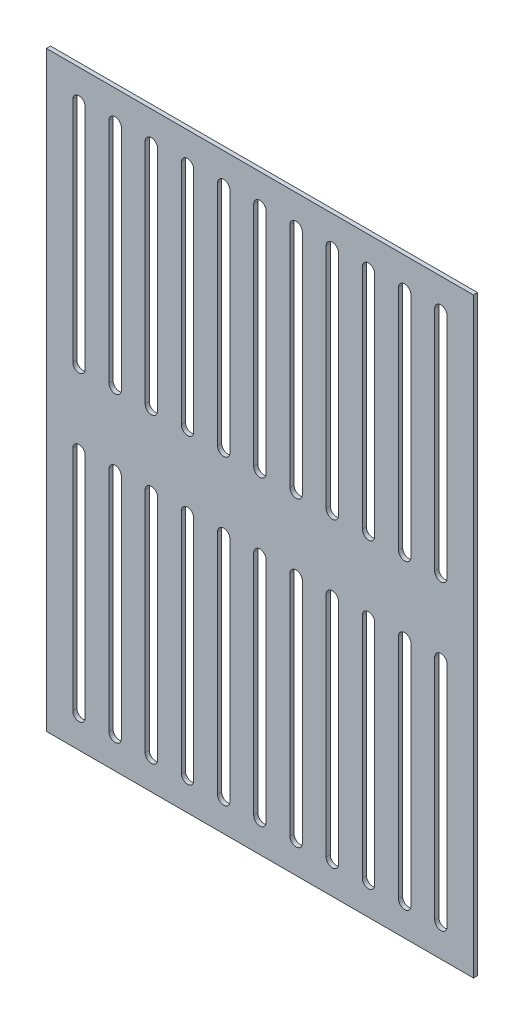
from build123d import *

# Parameters (mm, degrees)
SKETCH1_W           = 413
SKETCH1_H           = 572
BOSS_EXTRUDE1_DEPTH = 4
CUT_EXTRUDE1_DEPTH  = 4


with BuildPart() as part:
    # Sketch1 → Boss-Extrude1 (new body)
    with BuildSketch(Plane.XY):
        Rectangle(SKETCH1_W, SKETCH1_H)
    extrude(amount=BOSS_EXTRUDE1_DEPTH)

    # Sketch2 → Cut-Extrude1 (cut)
    with BuildSketch(Plane.XY.offset(4)):
        with BuildLine():
            Line((-99, -256), (-99, -36))
            ThreePointArc((-99, -36), (-105, -30), (-111, -36))
            Line((-111, -36), (-111, -256))
            ThreePointArc((-111, -256), (-105, -262), (-99, -256))
        make_face()
        with BuildLine():
            Line((-64, -256), (-64, -36))
            ThreePointArc((-64, -36), (-70, -30), (-76, -36))
            Line((-76, -36), (-76, -256))
            ThreePointArc((-76, -256), (-70, -262), (-64, -256))
        make_face()
        with BuildLine():
            Line((-29, -256), (-29, -36))
            ThreePointArc((-29, -36), (-35, -30), (-41, -36))
            Line((-41, -36), (-41, -256))
            ThreePointArc((-41, -256), (-35, -262), (-29, -256))
        make_face()
        with BuildLine():
            ThreePointArc((-6, -36), (0, -30), (6, -36))
            Line((6, -36), (6, -256))
            ThreePointArc((6, -256), (0, -262), (-6, -256))
            Line((-6, -256), (-6, -36))
        make_face()
        with BuildLine():
            ThreePointArc((29, -36), (35, -30), (41, -36))
            Line((41, -36), (41, -256))
            ThreePointArc((41, -256), (35, -262), (29, -256))
            Line((29, -256), (29, -36))
        make_face()
        with BuildLine():
            ThreePointArc((64, -36), (70, -30), (76, -36))
            Line((76, -36), (76, -256))
            ThreePointArc((76, -256), (70, -262), (64, -256))
            Line((64, -256), (64, -36))
        make_face()
        with BuildLine():
            ThreePointArc((169, -36), (175, -30), (181, -36))
            Line((181, -36), (181, -256))
            ThreePointArc((181, -256), (175, -262), (169, -256))
            Line((169, -256), (169, -36))
        make_face()
        with BuildLine():
            ThreePointArc((134, -36), (140, -30), (146, -36))
            Line((146, -36), (146, -256))
            ThreePointArc((146, -256), (140, -262), (134, -256))
            Line((134, -256), (134, -36))
        make_face()
        with BuildLine():
            ThreePointArc((99, -36), (105, -30), (111, -36))
            Line((111, -36), (111, -256))
            ThreePointArc((111, -256), (105, -262), (99, -256))
            Line((99, -256), (99, -36))
        make_face()
        with BuildLine():
            ThreePointArc((-169, 36), (-175, 30), (-181, 36))
            Line((-181, 36), (-181, 256))
            ThreePointArc((-181, 256), (-175, 262), (-169, 256))
            Line((-169, 256), (-169, 36))
        make_face()
        with BuildLine():
            ThreePointArc((-134, 36), (-140, 30), (-146, 36))
            Line((-146, 36), (-146, 256))
            ThreePointArc((-146, 256), (-140, 262), (-134, 256))
            Line((-134, 256), (-134, 36))
        make_face()
        with BuildLine():
            ThreePointArc((-99, 36), (-105, 30), (-111, 36))
            Line((-111, 36), (-111, 256))
            ThreePointArc((-111, 256), (-105, 262), (-99, 256))
            Line((-99, 256), (-99, 36))
        make_face()
        with BuildLine():
            ThreePointArc((-64, 36), (-70, 30), (-76, 36))
            Line((-76, 36), (-76, 256))
            ThreePointArc((-76, 256), (-70, 262), (-64, 256))
            Line((-64, 256), (-64, 36))
        make_face()
        with BuildLine():
            ThreePointArc((-29, 36), (-35, 30), (-41, 36))
            Line((-41, 36), (-41, 256))
            ThreePointArc((-41, 256), (-35, 262), (-29, 256))
            Line((-29, 256), (-29, 36))
        make_face()
        with BuildLine():
            Line((-6, 256), (-6, 36))
            ThreePointArc((-6, 36), (0, 30), (6, 36))
            Line((6, 36), (6, 256))
            ThreePointArc((6, 256), (0, 262), (-6, 256))
        make_face()
        with BuildLine():
            Line((64, 256), (64, 36))
            ThreePointArc((64, 36), (70, 30), (76, 36))
            Line((76, 36), (76, 256))
            ThreePointArc((76, 256), (70, 262), (64, 256))
        make_face()
        with BuildLine():
            Line((99, 256), (99, 36))
            ThreePointArc((99, 36), (105, 30), (111, 36))
            Line((111, 36), (111, 256))
            ThreePointArc((111, 256), (105, 262), (99, 256))
        make_face()
        with BuildLine():
            Line((134, 256), (134, 36))
            ThreePointArc((134, 36), (140, 30), (146, 36))
            Line((146, 36), (146, 256))
            ThreePointArc((146, 256), (140, 262), (134, 256))
        make_face()
        with BuildLine():
            Line((169, 256), (169, 36))
            ThreePointArc((169, 36), (175, 30), (181, 36))
            Line((181, 36), (181, 256))
            ThreePointArc((181, 256), (175, 262), (169, 256))
        make_face()
        with BuildLine():
            Line((-181, -256), (-181, -36))
            ThreePointArc((-181, -36), (-175, -30), (-169, -36))
            Line((-169, -36), (-169, -256))
            ThreePointArc((-169, -256), (-175, -262), (-181, -256))
        make_face()
        with BuildLine():
            Line((-146, -256), (-146, -36))
            ThreePointArc((-146, -36), (-140, -30), (-134, -36))
            Line((-134, -36), (-134, -256))
            ThreePointArc((-134, -256), (-140, -262), (-146, -256))
        make_face()
        with BuildLine():
            Line((29, 256), (29, 36))
            ThreePointArc((29, 36), (35, 30), (41, 36))
            Line((41, 36), (41, 256))
            ThreePointArc((41, 256), (35, 262), (29, 256))
        make_face()
    extrude(amount=-CUT_EXTRUDE1_DEPTH, mode=Mode.SUBTRACT)


solid = part.part
